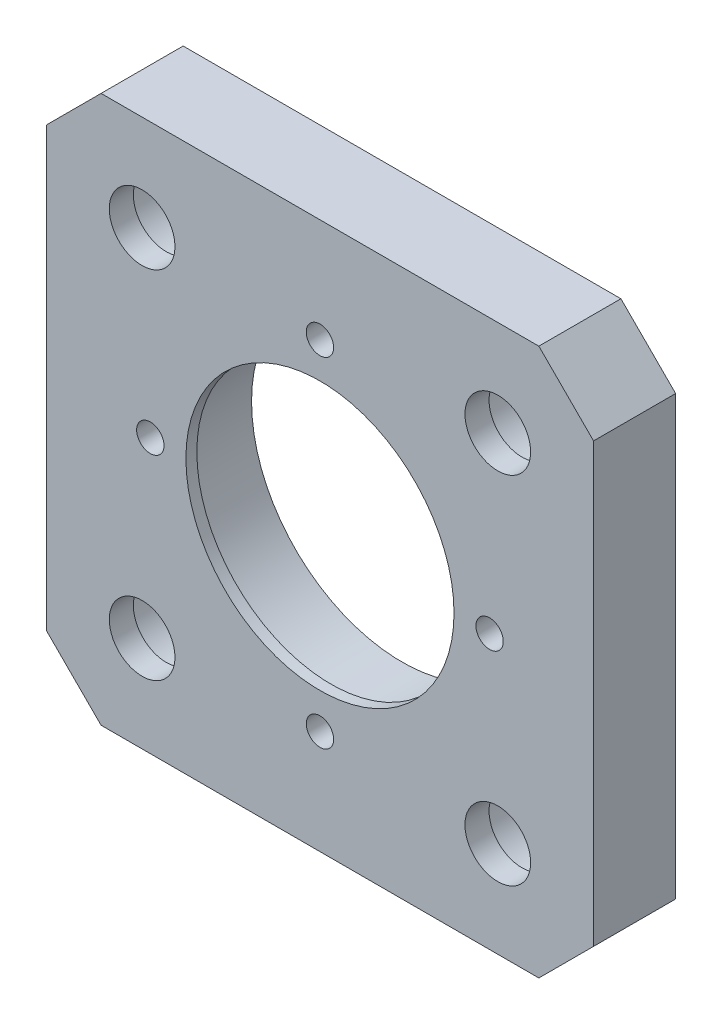
SolidWorks part; units mm, degrees
material "6061Al"
ref_plane "前视基准面" through (0, 0, 0) normal (0, 0, 1) x (1, 0, 0)
ref_plane "上视基准面" through (0, 0, 0) normal (0, 1, 0) x (1, 0, 0)
ref_plane "右视基准面" through (0, 0, 0) normal (1, 0, 0) x (0, 0, -1)
sketch "草图1" plane through (0, 0, 0) normal (0, 0, 1) x (1, 0, 0)
  line L1 (-50, -50) -> (50, -50)
  line L2 (-50, -50) -> (-50, 50)
  line L3 (-50, 50) -> (50, 50)
  line L4 (50, -50) -> (50, 50)
  line L5 (-50, -50) -> (50, 50) construction
  line L6 (-50, 50) -> (50, -50) construction
  point P0 (0, 0)
  dimension "D1" = 100
extrude "凸台-拉伸1" add sketch "草图1" along normal blind 15
hole_wizard "M10 六角凹头螺钉的柱形沉头孔1" positions "草图7" profile "草图8" counterbore size "M10" standard "ISO" end condition through all
sketch "草图7" plane through (0, 0, 0) normal (0, 0, -1) x (-1, 0, 0)
  line L0 (0, 0) -> (0, 50) construction
  line L1 (-50, 50) -> (50, 50) construction
  line L3 (0, 0) -> (50, 0) construction
  line L4 (50, 50) -> (50, -50) construction
  point P0 (-32.5, 32.5)
  point P17 (32.5, 32.5)
  point P18 (32.5, -32.5)
  point P19 (-32.5, -32.5)
  dimension "D1" = 65
  dimension "D2" = 65
sketch "草图8" plane through (32.5, 32.5, 0) normal (1, 0, 0) x (0, 1, 0)
  line L0 (0, 0) -> (0, 15)
  line L1 (0, 15) -> (6, 15)
  line L3 (6, 15) -> (6, 10.6)
  line L4 (6, 10.6) -> (9, 10.6)
  line L5 (9, 10.6) -> (9, 0)
  line L7 (9, 0) -> (0, 0)
  line L11 (0, -6.35) -> (0, 107.95) construction
  dimension "通孔孔直径" = 12
  dimension "通孔孔深度" = 15
  dimension "柱形沉头孔直径" = 18
  dimension "柱形沉头孔深度" = 10.6
chamfer "倒角1" distance 10 angle 45 4 edges at (50, -50, 7.5) (-50, -50, 7.5) (-50, 50, 7.5) (50, 50, 7.5)
sketch "草图11" plane through (0, 0, 0) normal (0, 0, -1) x (-1, 0, 0)
  circle A0 centre (0, 0) radius 27.5
  dimension "D1" = 55
extrude "切除-拉伸4" cut sketch "草图11" against normal blind 13
hole_wizard "M6 螺纹孔1" positions "草图12" profile "草图13" tap size "M6" standard "ISO"
sketch "草图12" plane through (0, 0, 0) normal (0, 0, -1) x (-1, 0, 0)
  line L0 (0, 0) -> (0, 31) construction
  line L1 (0, 0) -> (0, 31) construction
  circle A3 centre (0, 0) radius 27.5 construction
  point P0 (0, 31)
  point P17 (31, 0)
  point P18 (0, -31)
  point P19 (-31, 0)
  dimension "D1" = 3.5
  dimension "D2" = 4
sketch "草图13" plane through (0, 31, 0) normal (1, 0, 0) x (0, 1, 0)
  line L0 (0, 0) -> (0, 16.5022)
  line L1 (0, 16.5022) -> (2.5, 15)
  line L2 (2.5, 15) -> (2.5, 0)
  line L5 (2.5, 0) -> (0, 0)
  line L10 (0, 16.5022) -> (-2.5, 15) construction
  line L11 (0, -6.35) -> (0, 107.95) construction
  dimension "螺纹孔钻头直径" = 5
  dimension "螺纹孔钻头深度" = 15
  dimension "导头角度" = 118
cosmetic thread "孔螺蚊线5" parameters "D1"=12, "D2"=6
cosmetic thread "孔螺蚊线6" parameters "D1"=12, "D2"=6
cosmetic thread "孔螺蚊线7" parameters "D1"=12, "D2"=6
cosmetic thread "孔螺蚊线8" parameters "D1"=12, "D2"=6
sketch "草图14" plane through (0, 0, 13) normal (0, 0, -1) x (-1, 0, 0)
  circle A4 centre (0, 0) radius 24.5
  circle A5 centre (0, 0) radius 24.5
  dimension "D1" = 3
extrude "切除-拉伸5" cut sketch "草图14" against normal through all
